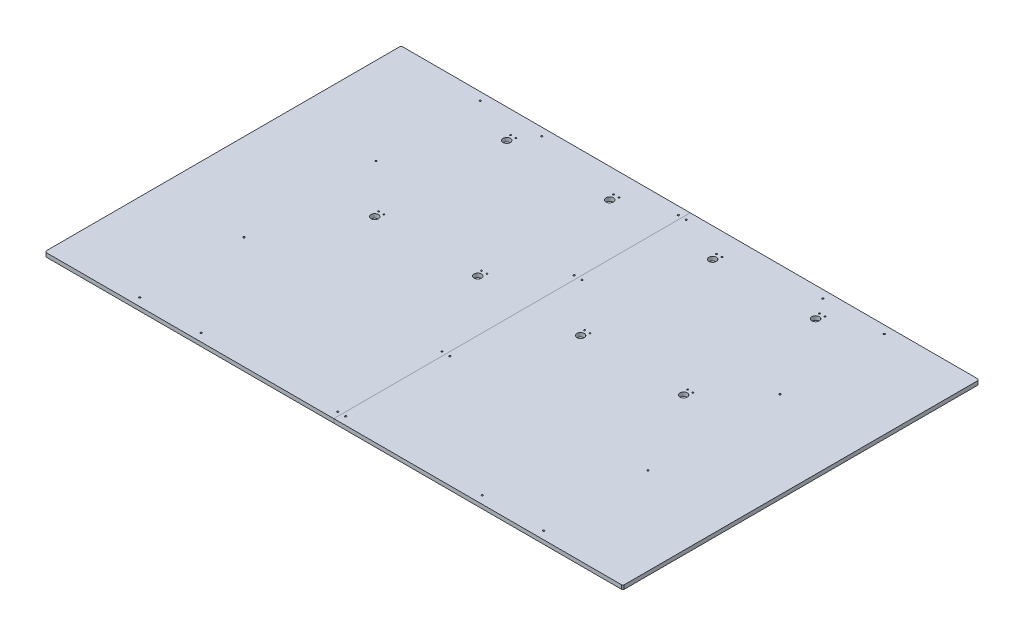
SolidWorks part; units mm, degrees
material "A6061"
ref_plane "前基準面" through (0, 0, 0) normal (0, 0, 1) x (1, 0, 0)
ref_plane "上基準面" through (0, 0, 0) normal (0, 1, 0) x (1, 0, 0)
ref_plane "右基準面" through (0, 0, 0) normal (1, 0, 0) x (0, 0, -1)
sketch "草图1" plane through (0, 0, 0) normal (0, 1, 0) x (1, 0, 0)
  line L1 (-1095, -675) -> (1095, -675)
  line L2 (-1095, -675) -> (-1095, 675)
  line L3 (-1095, 675) -> (1095, 675)
  line L4 (1095, -675) -> (1095, 675)
  line L5 (-1095, -675) -> (1095, 675) construction
  line L6 (-1095, 675) -> (1095, -675) construction
  point P0 (0, 0)
  dimension "D1" = 2190
  dimension "D2" = 1350
extrude "凸台-拉伸1" add sketch "草图1" along normal mid plane 15
chamfer "倒角1" distance 5 angle 45 4 edges at (1095, 0, -675) (1095, 0, 675) (-1095, 0, -675) (-1095, 0, 675)
hole_wizard "Ø25.0 (25) 直径孔1" positions "草图6" profile "草图7" hole size "Ø25.0" standard "GB" end condition through all
sketch "草图6" plane through (0, 7.5, 0) normal (0, 1, 0) x (1, 0, 0)
  line L0 (0, 787.4627) -> (0, 0) construction
  line L2 (1090, 675) -> (-1090, 675) construction
  point P0 (-585, 565)
  point P5 (-195, 565)
  point P6 (195, 565)
  point P7 (585, 565)
  point P20 (-585, 65)
  point P21 (-195, 65)
  point P22 (195, 65)
  point P23 (585, 65)
  dimension "D2" = 390
  dimension "D3" = 110
  dimension "D5" = 500
  dimension "D1" = 4
  dimension "D4" = 2
sketch "草图7" plane through (-585, 7.5, -565) normal (1, 0, 0) x (0, 0, 1)
  line L0 (0, 0) -> (0, 15)
  line L1 (0, 15) -> (14, 15)
  line L2 (14, 15) -> (14, 0)
  line L5 (14, 0) -> (0, 0)
  line L11 (0, -6.35) -> (0, 107.95) construction
  dimension "通孔孔直径" = 28
  dimension "通孔孔深度" = 15
hole_wizard "打孔尺寸(%根据)内六角圆柱头螺钉的类型2" positions "草图8" profile "草图9" counterbore size "M5" standard "GB" end condition through all
sketch "草图8" plane through (0, -7.5, 0) normal (0, 1, 0) x (1, 0, 0)
  line L1 (-585, 565) -> (-585, 631.3153) construction
  line L3 (-195, 565) -> (-195, 631.3153) construction
  line L4 (195, 565) -> (195, 631.3153) construction
  line L5 (585, 565) -> (585, 631.3153) construction
  line L6 (-195, 65) -> (-195, 131.3153) construction
  line L7 (195, 65) -> (195, 131.3153) construction
  line L8 (585, 65) -> (585, 131.3153) construction
  line L9 (-585, 65) -> (-585, 131.3153) construction
  point P0 (-595, 590)
  point P2 (-575, 590)
  point P14 (-205, 590)
  point P15 (-185, 590)
  point P18 (185, 590)
  point P19 (205, 590)
  point P22 (575, 590)
  point P23 (595, 590)
  point P26 (-205, 90)
  point P27 (-185, 90)
  point P30 (185, 90)
  point P31 (205, 90)
  point P34 (575, 90)
  point P35 (595, 90)
  point P38 (-595, 90)
  point P39 (-575, 90)
  dimension "D1" = 20
  dimension "D2" = 25
  dimension "D3" = 4
  dimension "D4" = 2
sketch "草图9" plane through (-595, -7.5, -590) normal (1, 0, 0) x (0, 0, -1)
  line L0 (0, 0) -> (0, 15)
  line L1 (0, 15) -> (2.75, 15)
  line L3 (2.75, 15) -> (2.75, 5.7)
  line L4 (2.75, 5.7) -> (5, 5.7)
  line L5 (5, 5.7) -> (5, 0)
  line L7 (5, 0) -> (0, 0)
  line L11 (0, -6.35) -> (0, 107.95) construction
  dimension "通孔孔直径" = 5.5
  dimension "通孔孔深度" = 15
  dimension "柱形沉头孔直径" = 10
  dimension "柱形沉头孔深度" = 5.7
hole_wizard "打孔尺寸(%根据)内六角圆柱头螺钉的类型3" positions "草图10" profile "草图11" counterbore size "M6" standard "GB" end condition through all
sketch "草图10" plane through (0, -7.5, 0) normal (0, -1, 0) x (-1, 0, 0)
  line L0 (0, 877.4584) -> (0, 0) construction
  line L1 (0, 0) -> (-1346.5612, 0) construction
  line L3 (-1095, -670) -> (-1095, 670) construction
  line L4 (-1090, 675) -> (1090, 675) construction
  point P0 (-765, 645)
  point P2 (-532.5, 645)
  point P4 (-765, 250)
  point P14 (15, 645)
  point P16 (15, 250)
  point P18 (765, 250)
  point P19 (532.5, 645)
  point P20 (765, 645)
  point P21 (765, -645)
  point P22 (532.5, -645)
  point P23 (765, -250)
  point P24 (15, -250)
  point P25 (15, -645)
  point P26 (-765, -250)
  point P27 (-532.5, -645)
  point P28 (-765, -645)
  point P37 (-15, -645)
  point P38 (-15, -250)
  point P39 (-15, 250)
  point P40 (-15, 645)
  dimension "D1" = 1065
  dimension "D2" = 330
  dimension "D3" = 30
  dimension "D4" = 500
  dimension "D5" = 30
sketch "草图11" plane through (765, -7.5, -645) normal (1, 0, 0) x (0, 0, -1)
  line L0 (0, 0) -> (0, 15)
  line L1 (0, 15) -> (3.3, 15)
  line L3 (3.3, 15) -> (3.3, 6.8)
  line L4 (3.3, 6.8) -> (5.5, 6.8)
  line L5 (5.5, 6.8) -> (5.5, 0)
  line L7 (5.5, 0) -> (0, 0)
  line L11 (0, -6.35) -> (0, 107.95) construction
  dimension "通孔孔直径" = 6.6
  dimension "通孔孔深度" = 15
  dimension "柱形沉头孔直径" = 11
  dimension "柱形沉头孔深度" = 6.8
sketch "草图12" plane through (0, 7.5, 0) normal (0, 1, 0) x (1, 0, 0)
  line L0 (0, 675) -> (0, -675)
  line L1 (1090, 675) -> (-1090, 675) construction
  line L2 (-1090, -675) -> (1090, -675) construction
split line "分割线1"
